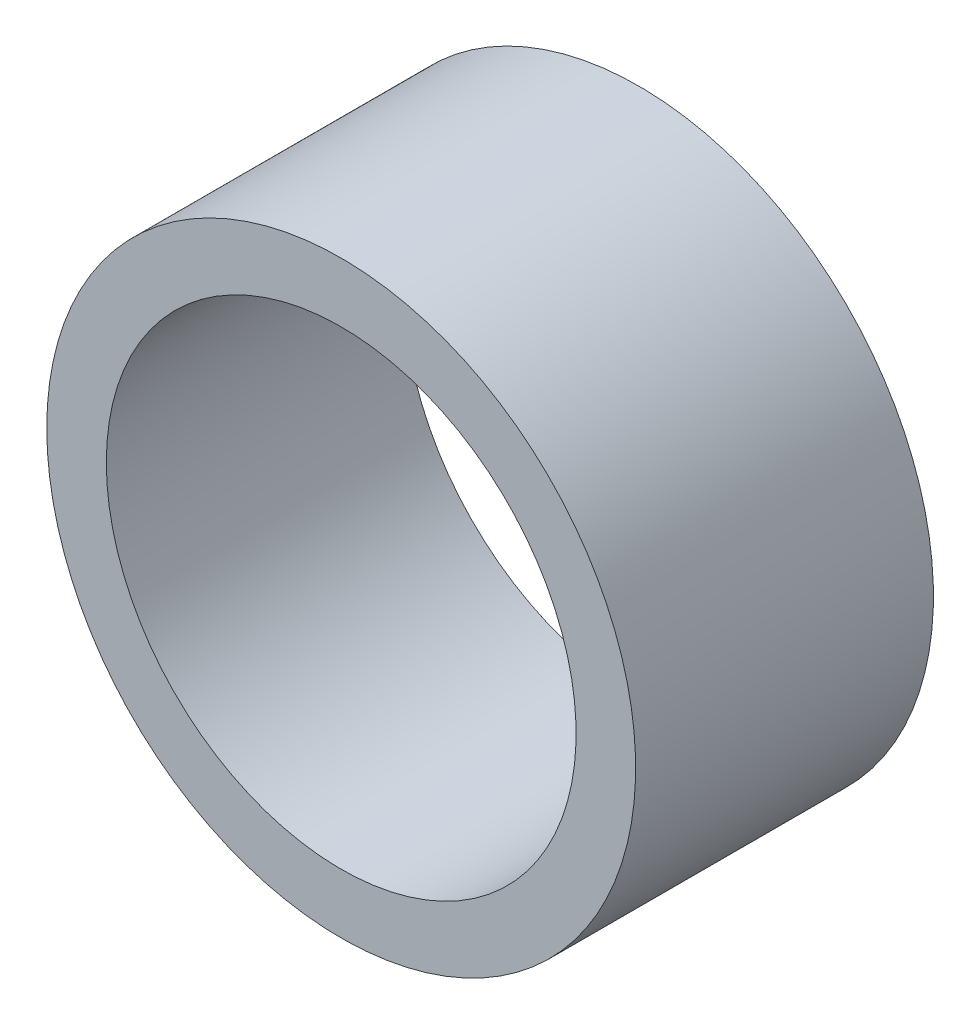
SolidWorks part; units mm, degrees
material "普通碳钢"
ref_plane "Front Plane" through (0, 0, 0) normal (0, 0, 1) x (1, 0, 0)
ref_plane "Top Plane" through (0, 0, 0) normal (0, 1, 0) x (1, 0, 0)
ref_plane "Right Plane" through (0, 0, 0) normal (1, 0, 0) x (0, 0, -1)
other "Configuration Table"
sketch "Sketch1" plane through (0, 0, 0) normal (0, 0, 1) x (1, 0, 0)
  circle A0 centre (0, 0) radius 35.5
  circle A1 centre (0, 0) radius 44.5
  dimension "D1" = 71
  dimension "D2" = 89
extrude "Boss-Extrude1" add sketch "Sketch1" along normal blind 45
